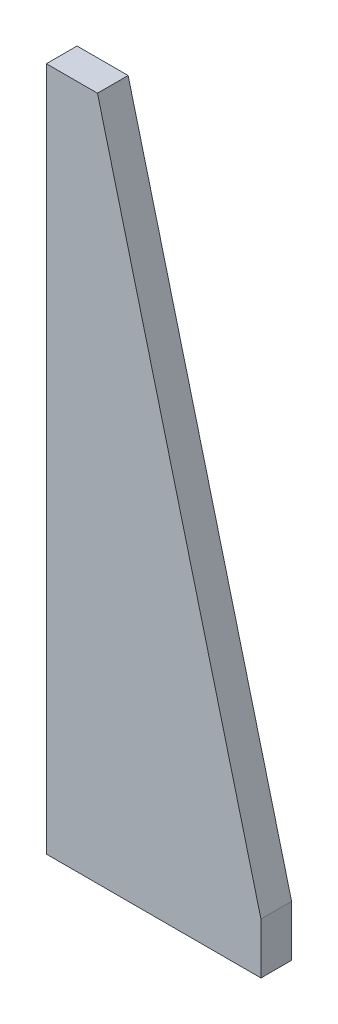
SolidWorks part; units mm, degrees
material "Q345"
ref_plane "前视基准面" through (0, 0, 0) normal (0, 0, 1) x (1, 0, 0)
ref_plane "上视基准面" through (0, 0, 0) normal (0, 1, 0) x (1, 0, 0)
ref_plane "右视基准面" through (0, 0, 0) normal (1, 0, 0) x (0, 0, -1)
sketch "草图1" plane through (0, 0, 0) normal (0, 0, 1) x (1, 0, 0)
  line L0 (0, 0) -> (0, 670)
  line L1 (0, 670) -> (50, 670)
  line L2 (50, 670) -> (210, 50)
  line L3 (210, 50) -> (210, 0)
  line L4 (210, 0) -> (0, 0)
  dimension "D1" = 670
  dimension "D2" = 50
  dimension "D3" = 50
  dimension "D4" = 210
extrude "凸台-拉伸1" add sketch "草图1" along normal blind 30
